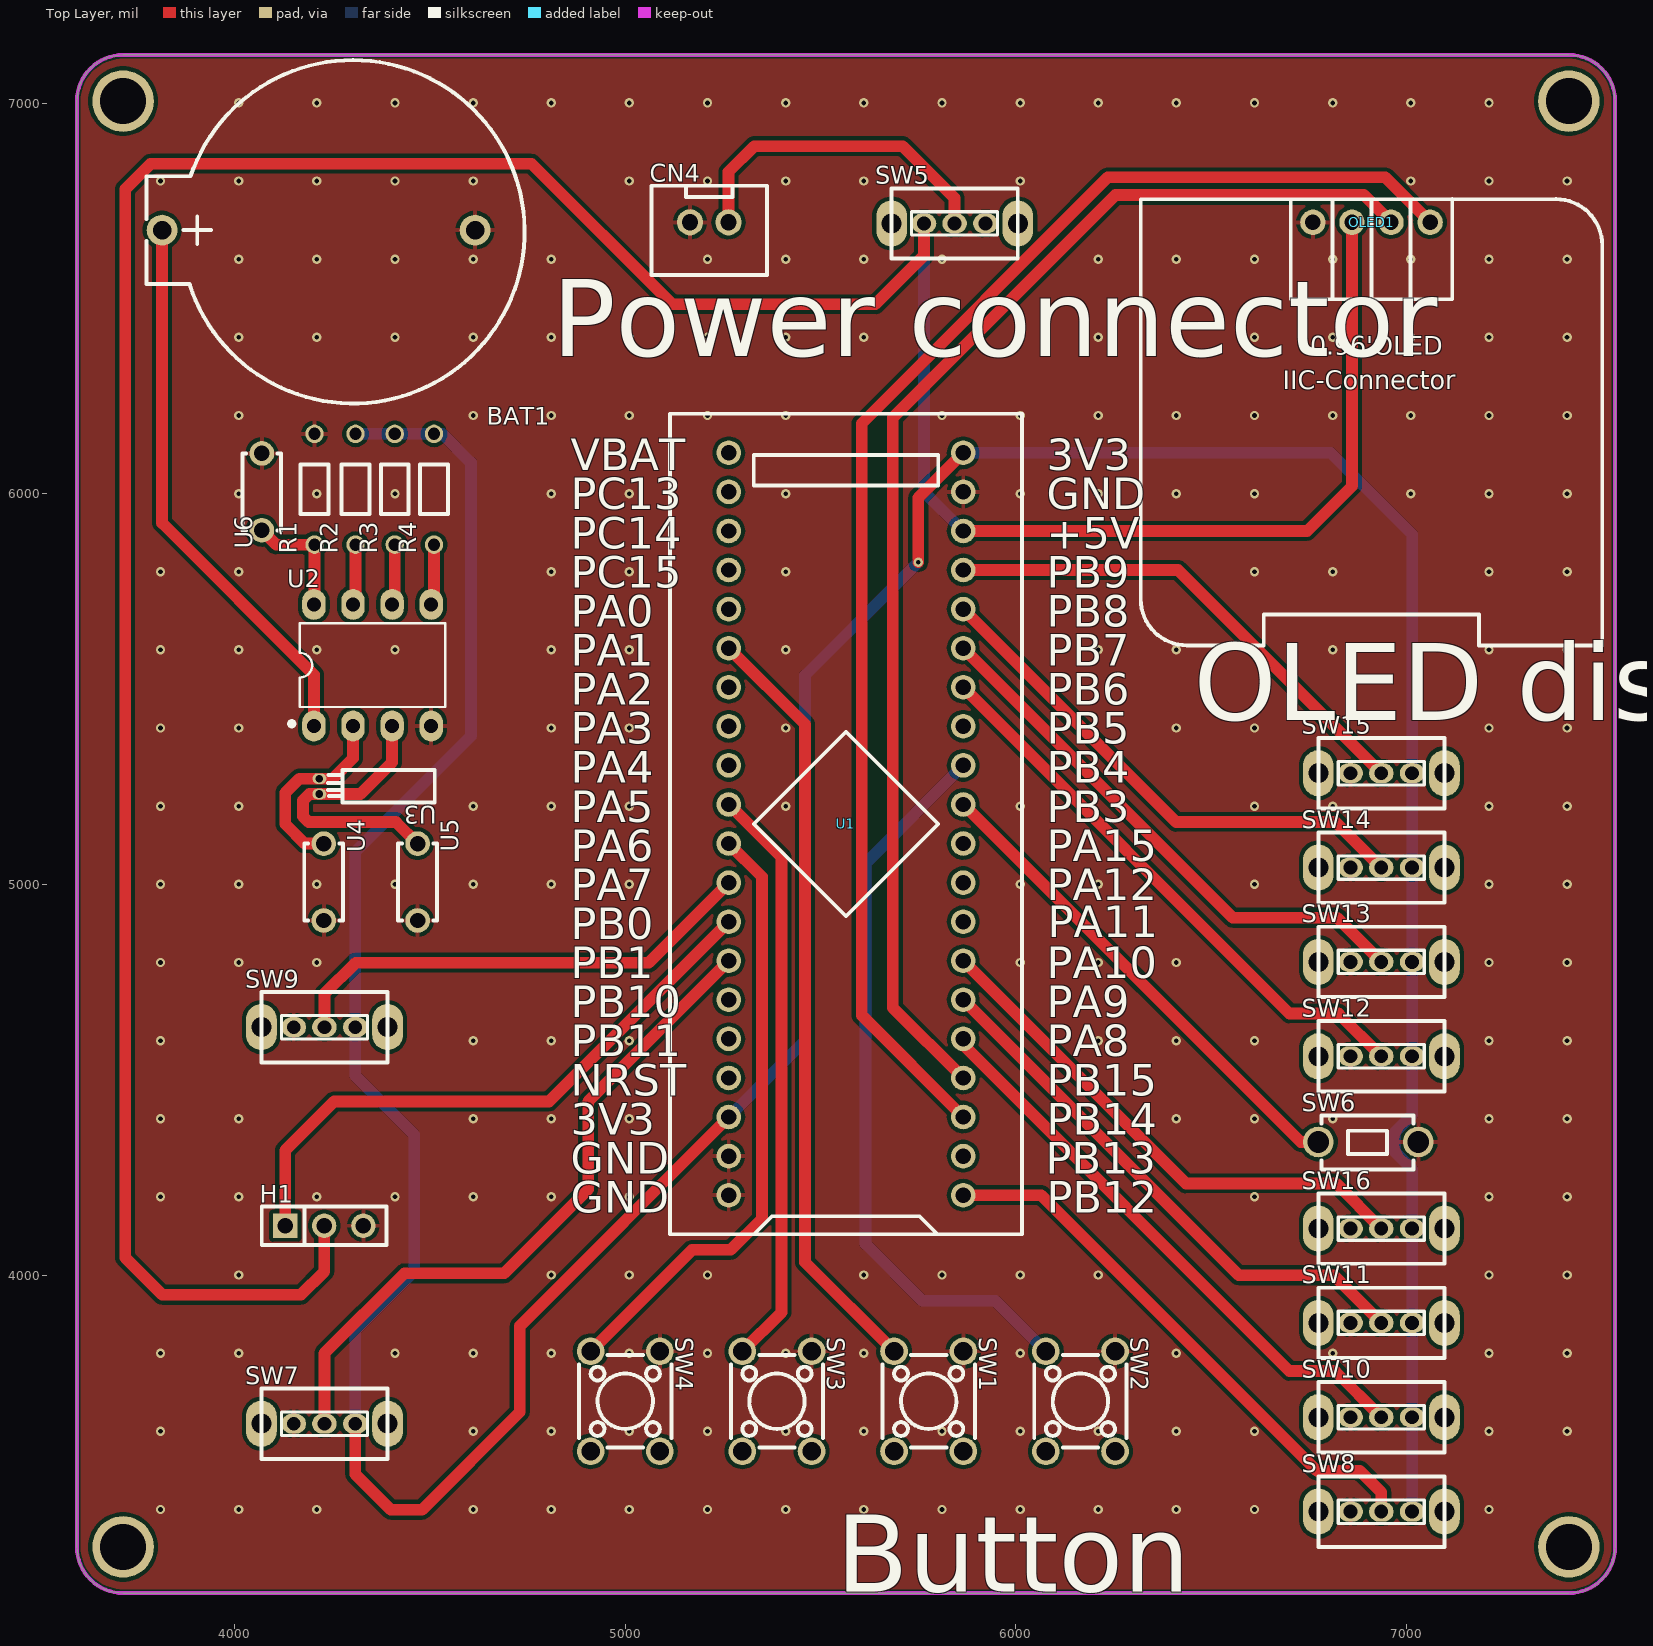
[diagram p0: Top Layer view]
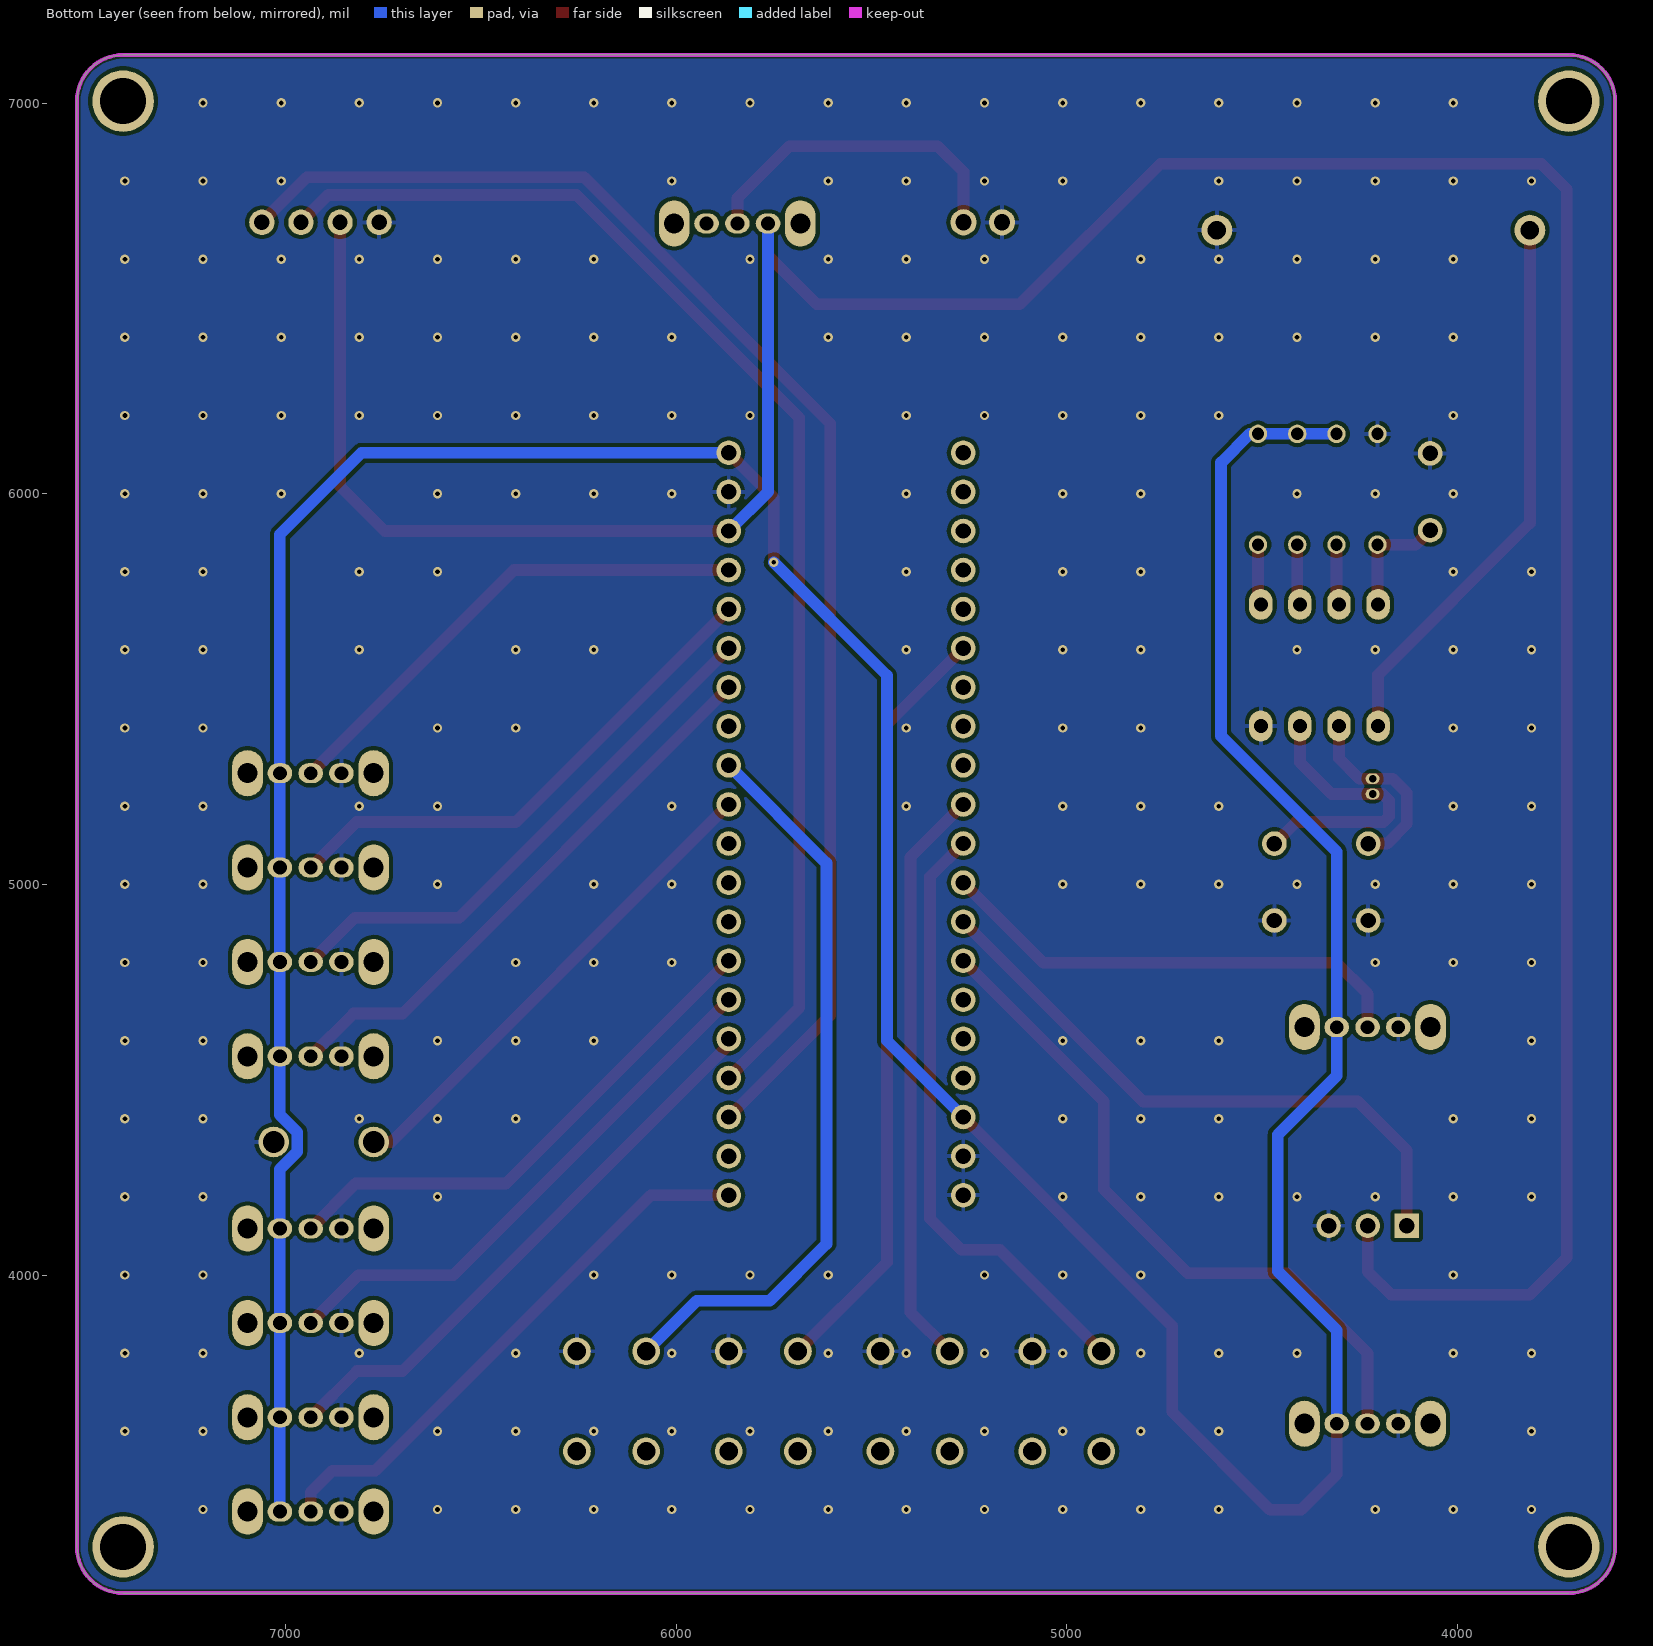
[diagram p1: Bottom Layer view, seen from below]
# Altium PCB MISC51813.pcbdoc
Units mil, origin at the board's own origin, x right, y up, seen from the top; angles counter-clockwise.
Board outline 3937.01 x 3937.01 mil, 2 copper layers (Top Layer, Bottom Layer), stack 62.206 mil thick; 30 components, 45 nets, 152 pads, 235 vias.

## Layer stack, top to bottom
Top Solder Mask Layer: solder mask 0.394, Dk 3.3
Top Layer: signal copper 1.379
Dielectric1: surface 59.449, FR4, Dk 4.5
Bottom Layer: signal copper 1.378
Bottom Solder Mask Layer: solder mask 0.394, Dk 3.3

## Board outline
3714.61,7123.5 ccw(c3714.61,7005.39) 3596.5,7005.39 3596.5,3304.61 ccw(c3714.61,3304.61) 3714.61,3186.5 7415.39,3186.5 ccw(c7415.39,3304.61) 7533.5,3304.61 7533.5,7005.39 ccw(c7415.39,7005.39) 7415.39,7123.5 3714.61,7123.5

## Design rules (kind name [scope] priority, off if disabled: settings)
BoardOutlineClearance copperThickness2oz_1 [All] p2 off: genericclearance=7.99 ignorepadtopadclearanceinfootprint=FALSE except(0: Arc-SplitContinuation Track-SplitContinuation SMDPad-SplitContinuation THPad-SplitContinuation Via-SplitContinuation Fill-SplitContinuation Region-SplitContinuation Poly-SplitContinuation Text-SplitContinuation Hole-SplitContinuation; 5.98: Arc-CutoutEdge Track-CutoutEdge SMDPad-CutoutEdge THPad-CutoutEdge Via-CutoutEdge Text-CutoutEdge; 6.9: Hole-OutlineEdge Hole-CutoutEdge; 10: Poly-OutlineEdge Poly-CutoutEdge; 11.81: Arc-OutlineEdge Track-OutlineEdge SMDPad-OutlineEdge THPad-OutlineEdge Via-OutlineEdge Fill-OutlineEdge Region-OutlineEdge Text-OutlineEdge Fill-CutoutEdge Region-CutoutEdge)
BoardOutlineClearance Plane_innerPlane_1 [All] p4 off: genericclearance=4.02 ignorepadtopadclearanceinfootprint=FALSE except(0: Arc-SplitContinuation Track-SplitContinuation SMDPad-SplitContinuation THPad-SplitContinuation Via-SplitContinuation Fill-SplitContinuation Region-SplitContinuation Poly-SplitContinuation Text-SplitContinuation Hole-SplitContinuation; 5.98: Arc-CutoutEdge Track-CutoutEdge SMDPad-CutoutEdge THPad-CutoutEdge Via-CutoutEdge Text-CutoutEdge; 6.9: Hole-OutlineEdge Hole-CutoutEdge; 10: Poly-OutlineEdge Poly-CutoutEdge; 11.81: Arc-OutlineEdge Track-OutlineEdge SMDPad-OutlineEdge THPad-OutlineEdge Via-OutlineEdge Fill-OutlineEdge Region-OutlineEdge Text-OutlineEdge Fill-CutoutEdge Region-CutoutEdge)
BoardOutlineClearance Copper_copperRegion_1 [All] p6 off: genericclearance=4.02 ignorepadtopadclearanceinfootprint=FALSE except(0: Arc-SplitContinuation Track-SplitContinuation SMDPad-SplitContinuation THPad-SplitContinuation Via-SplitContinuation Fill-SplitContinuation Region-SplitContinuation Poly-SplitContinuation Text-SplitContinuation Hole-SplitContinuation; 5.98: Arc-CutoutEdge Track-CutoutEdge SMDPad-CutoutEdge THPad-CutoutEdge Via-CutoutEdge Text-CutoutEdge; 6.9: Hole-OutlineEdge Hole-CutoutEdge; 10: Poly-OutlineEdge Poly-CutoutEdge; 11.81: Arc-OutlineEdge Track-OutlineEdge SMDPad-OutlineEdge THPad-OutlineEdge Via-OutlineEdge Fill-OutlineEdge Region-OutlineEdge Text-OutlineEdge Fill-CutoutEdge Region-CutoutEdge)
BoardOutlineClearance copperThickness1oz_1 [All] p8: genericclearance=4.02 ignorepadtopadclearanceinfootprint=FALSE except(0: Arc-SplitContinuation Track-SplitContinuation SMDPad-SplitContinuation THPad-SplitContinuation Via-SplitContinuation Fill-SplitContinuation Region-SplitContinuation Poly-SplitContinuation Text-SplitContinuation Hole-SplitContinuation; 5.98: Arc-CutoutEdge Track-CutoutEdge SMDPad-CutoutEdge THPad-CutoutEdge Via-CutoutEdge Text-CutoutEdge; 6.9: Hole-OutlineEdge Hole-CutoutEdge; 10: Poly-OutlineEdge Poly-CutoutEdge; 11.81: Arc-OutlineEdge Track-OutlineEdge SMDPad-OutlineEdge THPad-OutlineEdge Via-OutlineEdge Fill-OutlineEdge Region-OutlineEdge Text-OutlineEdge Fill-CutoutEdge Region-CutoutEdge)
Clearance copperThickness2oz [All] p1 off: gap=7.99 ignorepadtopadclearanceinfootprint=FALSE except(5.98: SMDPad-Track SMDPad-SMDPad THPad-Track SMDPad-THPad THPad-THPad Track-Via SMDPad-Via THPad-Via Via-Via Fill-SMDPad Region-SMDPad Fill-THPad Region-THPad Fill-Via Region-Via Fill-Fill Fill-Region Region-Region Arc-Track Arc-SMDPad Arc-THPad Arc-Via Fill-Arc Region-Arc Arc-Arc Text-Track SMDPad-Text Text-THPad Text-Via Fill-Text Region-Text Arc-Text Text-Text; 6.9: Hole-Track Hole-SMDPad Hole-THPad Hole-Via Fill-Hole Region-Hole Hole-Arc Hole-Text; 10: Poly-Track Poly-SMDPad Poly-THPad Poly-Via Poly-Fill Poly-Region Poly-Poly Poly-Arc Poly-Text Poly-Hole; 11.81: Fill-Track Region-Track)
Clearance Plane_innerPlane [All] p3 off: gap=4.02 ignorepadtopadclearanceinfootprint=FALSE except(5.98: SMDPad-Track SMDPad-SMDPad THPad-Track SMDPad-THPad THPad-THPad Track-Via SMDPad-Via THPad-Via Via-Via Fill-SMDPad Region-SMDPad Fill-THPad Region-THPad Fill-Via Region-Via Fill-Fill Fill-Region Region-Region Arc-Track Arc-SMDPad Arc-THPad Arc-Via Fill-Arc Region-Arc Arc-Arc Text-Track SMDPad-Text Text-THPad Text-Via Fill-Text Region-Text Arc-Text Text-Text; 6.9: Hole-Track Hole-SMDPad Hole-THPad Hole-Via Fill-Hole Region-Hole Hole-Arc Hole-Text; 10: Poly-Track Poly-SMDPad Poly-THPad Poly-Via Poly-Fill Poly-Region Poly-Poly Poly-Arc Poly-Text Poly-Hole; 11.81: Fill-Track Region-Track)
Clearance Copper_copperRegion [All] p5 off: gap=4.02 ignorepadtopadclearanceinfootprint=FALSE except(5.98: SMDPad-Track SMDPad-SMDPad THPad-Track SMDPad-THPad THPad-THPad Track-Via SMDPad-Via THPad-Via Via-Via Fill-SMDPad Region-SMDPad Fill-THPad Region-THPad Fill-Via Region-Via Fill-Fill Fill-Region Region-Region Arc-Track Arc-SMDPad Arc-THPad Arc-Via Fill-Arc Region-Arc Arc-Arc Text-Track SMDPad-Text Text-THPad Text-Via Fill-Text Region-Text Arc-Text Text-Text; 6.9: Hole-Track Hole-SMDPad Hole-THPad Hole-Via Fill-Hole Region-Hole Hole-Arc Hole-Text; 10: Poly-Track Poly-SMDPad Poly-THPad Poly-Via Poly-Fill Poly-Region Poly-Poly Poly-Arc Poly-Text Poly-Hole; 11.81: Fill-Track Region-Track)
Clearance copperThickness1oz [All] p7: gap=4.02 ignorepadtopadclearanceinfootprint=FALSE except(5.98: SMDPad-Track SMDPad-SMDPad THPad-Track SMDPad-THPad THPad-THPad Track-Via SMDPad-Via THPad-Via Via-Via Fill-SMDPad Region-SMDPad Fill-THPad Region-THPad Fill-Via Region-Via Fill-Fill Fill-Region Region-Region Arc-Track Arc-SMDPad Arc-THPad Arc-Via Fill-Arc Region-Arc Arc-Arc Text-Track SMDPad-Text Text-THPad Text-Via Fill-Text Region-Text Arc-Text Text-Text; 6.9: Hole-Track Hole-SMDPad Hole-THPad Hole-Via Fill-Hole Region-Hole Hole-Arc Hole-Text; 10: Poly-Track Poly-SMDPad Poly-THPad Poly-Via Poly-Fill Poly-Region Poly-Poly Poly-Arc Poly-Text Poly-Hole; 11.81: Fill-Track Region-Track)
DiffPairsRouting differentialPair [All] p1: maxlimit=6 minlimit=6 mostfreqgap=6 toplayer_minwidth=5 toplayer_prefwidth=10 toplayer_maxwidth=100 toplayer_mingap=6 toplayer_prefgap=6 toplayer_maxgap=6 bottomlayer_minwidth=5 bottomlayer_prefwidth=10 bottomlayer_maxwidth=100 bottomlayer_mingap=6 bottomlayer_prefgap=6 bottomlayer_maxgap=6 maxuncoupledlength=10
HoleToHoleClearance otherClearance [All] p1: gap=11.81 allowstackedmicrovias=TRUE
Length netLength [All] p1: minlimit=0 maxlimit=0
PasteMaskExpansion pasteMaskExpansion [All] p1: expansion=0
PlaneConnect innerPlane [All] p1: planeconnectstyle=Relief reliefexpansion=20 reliefentries=4 reliefconductorwidth=10 reliefairgap=10
PolygonConnect copperRegion [All] p1: connectstyle=Relief reliefconductorwidth=10 reliefentries=4 polygonreliefangle="90 Angle" airgapwidth=10 via.connectstyle=Relief via.reliefconductorwidth=10 via.reliefentries=4 via.polygonreliefangle="90 Angle" via.airgapwidth=10
RoutingVias viaSize [All] p1: holewidth=12.01 width=24.02 viastyle="Through Hole" minholewidth=11.81 minwidth=19.68 maxholewidth=248.03 maxwidth=393.7
SolderMaskExpansion solderMaskExpansion [IsVia] p1: expansion=-1000 istentingtop=TRUE
SolderMaskExpansion solderMaskExpansion [All] p2: expansion=2 istentingtop=FALSE
Width copperThickness2oz_2 [All] p1 off: maxlimit=100 minlimit=8 preferedwidth=10
Width copperThickness1oz_2 [All] p2: maxlimit=100 minlimit=5 preferedwidth=10

## Components (designator, comment, footprint, x,y, rotation, side; value= is the part's Value field where it differs from the comment)
BAT1 "CR2032-2-1" BAT-TH_CR2032-2-1 4215,6675 r180 top
CN4 "XH2.54*2P_through-hole" CONN-TH_2P-P2.50-XH2.54-2P 5215,6695 r0 top
H1 "" HDR-TH_3P-P2.54-V-F 4229.55,4126.75 r0 top
OLED1 "" 0.96OLED_4P 6910,6695 r0 top
R1 "10kΩ" Res_1/8W 4207.19,6011.78 r90 top
R2 "10kΩ" Res_1/8W 4312.02,6011.78 r90 top
R3 "10kΩ" Res_1/8W 4412.5,6011.78 r90 top
R4 "10kΩ" Res_1/8W 4512.99,6011.78 r90 top
SW1 "" SW-TH_4P-L6.0-W6.0-P4.50-LS6.5 5776.67,3677.47 r270 top
SW2 "" SW-TH_4P-L6.0-W6.0-P4.50-LS6.5 6165,3677.47 r270 top
SW3 "" SW-TH_4P-L6.0-W6.0-P4.50-LS6.5 5388.33,3677.47 r270 top
SW4 "" SW-TH_4P-L6.0-W6.0-P4.50-LS6.5 5000,3677.47 r270 top
SW5 "" 拨动开关 5837.9,6692.05 r0 top
SW6 "" Key_TH_3.5x6x4.3 6895.34,4341.1 r0 top
SW7 "" 拨动开关 4225,3620 r0 top
SW8 "" 拨动开关 6930,3395 r0 top
SW9 "" 拨动开关 4225,4635 r0 top
SW10 "" 拨动开关 6930,3636.53 r0 top
SW11 "" 拨动开关 6930,3878.05 r0 top
SW12 "" 拨动开关 6930,4560.43 r0 top
SW13 "" 拨动开关 6930,4801.95 r0 top
SW14 "" 拨动开关 6930,5043.48 r0 top
SW15 "" 拨动开关 6930,5285 r0 top
SW16 "" 拨动开关 6930,4119.57 r0 top
U1 "STM32F103C8T6-Card" CONN-TH_L53.3-W22.9_STM32F103C8T6-CARD 5565,5155 r90 top
U2 "DS1302N(LX)" PDIP-8_L9.3-W6.4-P2.54-LS7.9-BL-1 4353.22,5561.4 r0 top
U3 "32.768kHz" CRYSTAL-TH_BD2.1-P0.70-D0.3 4217.19,5251.38 r180 top
U4 "30pF" CAP-TH_L5.0-W2.5-P5.00-D1.0 4228.48,5006.4 r270 top
U5 "30pF" CAP-TH_L5.0-W2.5-P5.00-D1.0 4468.48,5006.4 r270 top
U6 "1nF" CAP-TH_L5.0-W2.5-P5.00-D1.0 4070,6005 r270 top

## Footprints (in the part's own frame and the unit in brackets; to place one, negate y for a bottom-side part, rotate by r counter-clockwise, add the part's x,y. Pads: shape width x height; smd on the part's side, far side on the other; paste and mask are expansions set on the pad)
0.96OLED_4P [mm]
  round 1.65 hole 1 copper offset 0,0: 1(-3.81,-0.001) 2(-1.27,0.002) 3(1.27,0.002) 4(3.81,0.002)
  silkscreen extent -15,-27.5 15,1.5
BAT-TH_CR2032-2-1 [mm]
  round 2 hole 1.2: 1(10.175,0) 2(-10.175,0)
  silkscreen extent -13.4,-11.05 11.17,11.26
CAP-TH_L5.0-W2.5-P5.00-D1.0 [mm]
  round 1.6 hole 1: 1(-2.5,0) 2(2.5,0)
  silkscreen extent -2.5,-1.27 2.5,1.25
CONN-TH_2P-P2.50-XH2.54-2P [mm]
  round 1.7 hole 1.05 paste+0 mask+0.05: 1(1.25,0) 2(-1.25,0)
  silkscreen extent -3.75,-3.42 3.75,2.37
CONN-TH_L53.3-W22.9_STM32F103C8T6-CARD [mm]
  round 1.6 hole 1: 1(-24.13,-7.62) 2(-21.59,-7.62) 3(-19.05,-7.62) 4(-16.51,-7.62) 5(-13.97,-7.62) 6(-11.43,-7.62) 7(-8.89,-7.62) 8(-6.35,-7.62) 9(-3.81,-7.62) 10(-1.27,-7.62) 11(1.27,-7.62) 12(3.81,-7.62) 13(6.35,-7.62) 14(8.89,-7.62) 15(11.43,-7.62) 16(13.97,-7.62) 17(16.51,-7.62) 18(19.05,-7.62) 19(21.59,-7.62) 20(24.13,-7.62) 21(24.13,7.62) 22(21.59,7.62) 23(19.05,7.62) 24(16.51,7.62) 25(13.97,7.62) 26(11.43,7.62) 27(8.89,7.62) 28(6.35,7.62) 29(3.81,7.62) 30(1.27,7.62) 31(-1.27,7.62) 32(-3.81,7.62) 33(-6.35,7.62) 34(-8.89,7.62) 35(-11.43,7.62) 36(-13.97,7.62) 37(-16.51,7.62) 38(-19.05,7.62) 39(-21.59,7.62) 40(-24.13,7.62)
  silkscreen extent -26.67,-11.43 26.67,11.43
CRYSTAL-TH_BD2.1-P0.70-D0.3 [mm]
  oval 0.9x0.7 hole 0.5 paste+0 mask+0.05: 1(0,0.5) 2(0,-0.5)
  silkscreen extent -7.5,-1.05 -0.57,1.05
HDR-TH_3P-P2.54-V-F [mil]
  rect 62x62 hole 40.16: 1(-100,0)
  round 62 hole 40.16: 2(0,0) 3(100,0)
  silkscreen extent -160,-49 160,49
Key_TH_3.5x6x4.3 [mil]
  round 78.7 hole 55.1 paste+0 mask+2: A(-121.44,0) B(134.46,0)
  silkscreen extent -114,-70 123,68
PDIP-8_L9.3-W6.4-P2.54-LS7.9-BL-1 [mm]
  oval 1.524x2 hole 0.9: 1(-3.81,-3.95) 2(-1.27,-3.95) 3(1.27,-3.95) 4(3.81,-3.95) 5(3.81,3.95) 6(1.27,3.95) 7(-1.27,3.95) 8(-3.81,3.95)
  silkscreen extent -5.4,-3.95 4.73,2.72
Res_1/8W [mil]
  round 47.2 hole 31.5 paste+0 mask+2: 1(-141.7,2.48) 2(141.7,2.48)
  silkscreen extent -63,-33 63,38
SW-TH_4P-L6.0-W6.0-P4.50-LS6.5 [mm]
  round 1.8 hole 1.2: 1(-3.25,2.25) 2(3.25,2.25) 3(-3.25,-2.25) 4(3.25,-2.25)
  silkscreen extent -3,-3 3,3
拨动开关 [mil]
  oval 63x51.2 hole 35.4 paste+0 mask+2: 1(-73.4,0) 2(5,0) 3(84,0)
  oval 78.7x118.1 hole 51.2 paste+0 mask+2: 4(166.7,0) 5(-156.1,0)
  silkscreen extent -156,-90 167,90

## Free pads (board coordinates)
  round 157.48 hole 118.11: 1(3714.61,7005.39) 1(3714.61,3304.61) 1(7415.39,7005.39) 1(7415.39,3304.61)

## Via types
v1: diameter 24.02, hole 12, Top Layer to Bottom Layer, 235 vias

## Nets (pads, with @x,y where several pads share a name; then routed paths per layer and width w, separated by ;. In a path a pad name is that pad's centre, name@x,y a point inside that pad or via, vN(x,y) a via of type N, cw(c..) or ccw(c..) an arc to the next point about the centre after c; other vN are vias at no path point)
$1N17118: CN4.1 SW5.2 | length 855.2
  Top Layer w30: CN4.1 5264.22,6824.22 5330,6890 5710,6890 5842.9,6757.1 SW5.2
$1N17188: U2.2 U3.2 U4.1 | length 491.7
  Top Layer w30: U4.1 4180.17,5104.83 4130,5155 4130,5235 4166.06,5271.06 U3.2 4251.06,5271.06 4303.22,5323.22 U2.2
$1N17189: U2.3 U3.1 U5.1 | length 724.1
  Top Layer w30: U2.3 4403.22,5313.22 4321.69,5231.69 U3.1 4191.69,5231.69 4175,5215 4175,5175 4190,5160 4413.31,5160 U5.1
$1N17190: BAT1.1 U2.1 | length 1430.2
  Top Layer w30: BAT1.1 3814.41,5925.59 4203.22,5536.78 U2.1
$1N17194: R1.1 U2.8 U6.2 | length 303.6
  Top Layer w30: U6.2 4106.49,5870.08 R1.1 4204.71,5718.41 U2.8
$1N17199: R4.1 U2.5 | length 156.2
  Top Layer w30: U2.5 4510.51,5724.2 R4.1
$1N17200: R3.1 U2.6 | length 156
  Top Layer w30: U2.6 4410.02,5723.72 R3.1
$1N17201: R2.1 U2.7 | length 155.8
  Top Layer w30: U2.7 4309.54,5723.23 R2.1
+5V: H1.2 OLED1.2 SW5.1 U1.18 | length 8326.8
  Top Layer w30: H1.2 4229.55,4009.55 4170,3950 3815,3950 3720,4045 3720,6780 3785,6845 4760,6845 5120,6485 5640,6485 5764.5,6609.5 SW5.1 ; U1.18 6745,5905 6860,6020 OLED1.2@6860,6695.05
  Bottom Layer w30: SW5.1 5764.5,6005.5 U1.18
GND: BAT1.2 CN4.2 H1.3 OLED1.1 R1.2 SW1.1 SW2.1 SW3.1 SW4.1 SW6.B SW7.1 SW8.1 SW9.1 SW10.1 SW11.1 SW12.1 SW13.1 SW14.1 SW15.1 SW16.1 U1.19 U1.39 U1.40 U2.4 U4.2 U5.2 U6.1
  other v1: 3810.6,3400.6 4010.6,3400.6 4210.6,3400.6 4610.6,3400.6 4810.6,3400.6 5010.6,3400.6 5210.6,3400.6 5410.6,3400.6 5610.6,3400.6 5810.6,3400.6 6010.6,3400.6 6210.6,3400.6 6410.6,3400.6 6610.6,3400.6 7210.6,3400.6 3810.6,3600.6 4610.6,3600.6 4810.6,3600.6 5010.6,3600.6 5210.6,3600.6 5410.6,3600.6 5610.6,3600.6 5810.6,3600.6 6010.6,3600.6 6210.6,3600.6 6410.6,3600.6 6610.6,3600.6 7210.6,3600.6 7410.6,3600.6 3810.6,3800.6 4010.6,3800.6 4410.6,3800.6 4610.6,3800.6 4810.6,3800.6 5010.6,3800.6 5210.6,3800.6 5410.6,3800.6 5610.6,3800.6 6010.6,3800.6 6410.6,3800.6 6810.6,3800.6 7210.6,3800.6 7410.6,3800.6 4010.6,4000.6 4810.6,4000.6 5010.6,4000.6 5210.6,4000.6 5610.6,4000.6 5810.6,4000.6 6010.6,4000.6 6210.6,4000.6 7210.6,4000.6 7410.6,4000.6 3810.6,4200.6 4010.6,4200.6 4210.6,4200.6 4410.6,4200.6 4610.6,4200.6 4810.6,4200.6 5010.6,4200.6 6610.6,4200.6 7210.6,4200.6 7410.6,4200.6 3810.6,4400.6 4010.6,4400.6 4610.6,4400.6 4810.6,4400.6 5010.6,4400.6 6410.6,4400.6 6610.6,4400.6 6810.6,4400.6 7210.6,4400.6 7410.6,4400.6 3810.6,4600.6 4610.6,4600.6 4810.6,4600.6 5010.6,4600.6 6210.6,4600.6 6410.6,4600.6 6610.6,4600.6 7210.6,4600.6 7410.6,4600.6 3810.6,4800.6 4010.6,4800.6 4210.6,4800.6 6010.6,4800.6 6210.6,4800.6 6410.6,4800.6 7210.6,4800.6 7410.6,4800.6 3810.6,5000.6 4010.6,5000.6 4210.6,5000.6 4410.6,5000.6 4610.6,5000.6 4810.6,5000.6 5010.6,5000.6 6010.6,5000.6 6210.6,5000.6 6610.6,5000.6 7210.6,5000.6 7410.6,5000.6 3810.6,5200.6 4010.6,5200.6 4610.6,5200.6 4810.6,5200.6 5010.6,5200.6 5410.6,5200.6 6010.6,5200.6 6610.6,5200.6 6810.6,5200.6 7210.6,5200.6 7410.6,5200.6 3810.6,5400.6 4010.6,5400.6 4810.6,5400.6 5010.6,5400.6 5410.6,5400.6 6410.6,5400.6 6610.6,5400.6 7210.6,5400.6 7410.6,5400.6 3810.6,5600.6 4010.6,5600.6 4210.6,5600.6 4410.6,5600.6 4810.6,5600.6 5010.6,5600.6 5410.6,5600.6 6210.6,5600.6 6410.6,5600.6 6810.6,5600.6 7210.6,5600.6 7410.6,5600.6 3810.6,5800.6 4010.6,5800.6 4810.6,5800.6 5010.6,5800.6 5410.6,5800.6 6610.6,5800.6 6810.6,5800.6 7210.6,5800.6 7410.6,5800.6 4010.6,6000.6 4210.6,6000.6 4410.6,6000.6 4810.6,6000.6 5010.6,6000.6 5410.6,6000.6 6010.6,6000.6 6210.6,6000.6 6410.6,6000.6 6610.6,6000.6 7010.6,6000.6 7210.6,6000.6 7410.6,6000.6 4010.6,6200.6 4610.6,6200.6 4810.6,6200.6 5010.6,6200.6 5210.6,6200.6 5410.6,6200.6 5810.6,6200.6 6010.6,6200.6 6210.6,6200.6 6410.6,6200.6 6610.6,6200.6 6810.6,6200.6 7010.6,6200.6 7210.6,6200.6 7410.6,6200.6 4010.6,6400.6 4210.6,6400.6 4410.6,6400.6 4610.6,6400.6 4810.6,6400.6 5010.6,6400.6 5210.6,6400.6 5410.6,6400.6 5610.6,6400.6 6010.6,6400.6 6210.6,6400.6 6410.6,6400.6 6610.6,6400.6 6810.6,6400.6 7010.6,6400.6 7210.6,6400.6 7410.6,6400.6 4010.6,6600.6 4210.6,6600.6 4410.6,6600.6 4610.6,6600.6 4810.6,6600.6 5210.6,6600.6 5410.6,6600.6 5610.6,6600.6 5810.6,6600.6 6210.6,6600.6 6410.6,6600.6 6610.6,6600.6 6810.6,6600.6 7010.6,6600.6 7210.6,6600.6 7410.6,6600.6 3810.6,6800.6 4010.6,6800.6 4210.6,6800.6 4410.6,6800.6 4610.6,6800.6 5010.6,6800.6 5210.6,6800.6 5410.6,6800.6 5610.6,6800.6 6010.6,6800.6 7010.6,6800.6 7210.6,6800.6 7410.6,6800.6 4010.6,7000.6 4210.6,7000.6 4410.6,7000.6 4610.6,7000.6 4810.6,7000.6 5010.6,7000.6 5210.6,7000.6 5410.6,7000.6 5610.6,7000.6 5810.6,7000.6 6010.6,7000.6 6210.6,7000.6 6410.6,7000.6 6610.6,7000.6 6810.6,7000.6 7010.6,7000.6 7210.6,7000.6
NRST: U1.37
PA0: U1.25
PA1: SW1.3 U1.26 | length 1974.8
  Top Layer w30: U1.26 5460,5410 5460,4033.51 SW1.3
PA2: U1.27
PA3: U1.28
PA4: U1.29
PA5: SW3.3 U1.30 | length 1497
  Top Layer w30: U1.30 5400,5070 5400,3905.67 SW3.3
PA6: SW4.3 U1.31 | length 1574.4
  Top Layer w30: SW4.3 5171,4065 5270,4065 5350,4145 5350,5020 U1.31
PA7: SW9.2 U1.32 | length 1238.1
  Top Layer w30: SW9.2 4230,4720 4310,4800 5060,4800 U1.32
PA8: SW10.2 U1.5 | length 1479.9
  Top Layer w30: U1.5 5865,4590 6700,3755 6816.52,3755 SW10.2
PA9: SW11.2 U1.6 | length 1412.5
  Top Layer w30: U1.6 6570,4000 6813.05,4000 SW11.2
PA10: SW16.2 U1.7 | length 1353.9
  Top Layer w30: U1.7 6435,4235 6819.57,4235 SW16.2
PA11: U1.8
PA12: U1.9
PA15: U1.10
PB0: H1.1 U1.33 | length 1570.8
  Top Layer w30: H1.1 4129.55,4319.55 4255,4445 4805,4445 U1.33
PB1: SW7.2 U1.34 | length 1763.1
  Top Layer w30: SW7.2 4230,3800 4435,4005 4690,4005 4905,4220 4905,4445 U1.34
PB3: SW6.A U1.11 | length 1266.7
  Top Layer w30: U1.11 6728.9,4341.1 SW6.A
PB4: SW2.3 U1.12 | length 1903.7
  Bottom Layer w30: U1.12 5615,5055 5615,4080 5760,3935 5946.84,3935 SW2.3
PB5: U1.13
PB6: SW12.2 U1.14 | length 1461.3
  Top Layer w30: U1.14 6700,4670 6825.43,4670 SW12.2
PB7: SW13.2 U1.15 | length 1402.6
  Top Layer w30: U1.15 6555,4915 6821.95,4915 SW13.2
PB8: SW14.2 U1.16 | length 1344
  Top Layer w30: U1.16 6410,5160 6818.48,5160 SW14.2
PB9: SW15.2 U1.17 | length 1285.4
  Top Layer w30: U1.17 6415,5805 SW15.2
PB10: U1.35
PB11: U1.36
PB12: SW8.2 U1.1 | length 1434.8
  Top Layer w30: U1.1 6065,4205 6770,3500 6880,3500 6935,3445 SW8.2
PB13: U1.2
PB14: OLED1.4 U1.3 | length 3646.3
  Top Layer w30: U1.3 5605,4665 5605,6180 6235,6810 6945.05,6810 OLED1.4@7060,6695.05
PB15: OLED1.3 U1.4 | length 3304.6
  Top Layer w30: U1.4 5685,4685 5685,6195 6255,6765 6890.05,6765 OLED1.3@6960,6695.05
PC13: U1.22
PC14: U1.23
PC15: U1.24
VBAT: U1.21
VCC: R2.2 R3.2 R4.2 SW7.3 SW8.3 SW9.3 SW10.3 SW11.3 SW12.3 SW13.3 SW14.3 SW15.3 SW16.3 U1.20 U1.38 | length 10423.4
  Top Layer w30: SW7.3 4309,3491 4400,3400 4480,3400 4730,3650 4730,3870 U1.38 ; v1(5750,5825) 5750,5990 U1.20
  Bottom Layer w30: SW7.3 4309,3859 4460,4010 4460,4360 4309,4511 SW9.3 4309,5084 4605,5380 4605,6080 4531.52,6153.48 R4.2 R3.2 R2.2 ; U1.38 5460,4600 5460,5535 v1(5750,5825) ; U1.20 6805,6105 7014,5896 SW15.3 SW14.3 SW13.3 SW12.3 7014,4410.63 6969.47,4366.09 6969.47,4316.11 7014,4271.57 SW16.3 SW11.3 SW10.3 SW8.3
pads on no net: SW1.2 SW1.4 SW2.2 SW2.4 SW3.2 SW3.4 SW4.2 SW4.4 SW5.3 SW5.4 SW5.5 SW7.4 SW7.5 SW8.4 SW8.5 SW9.4 SW9.5 SW10.4 SW10.5 SW11.4 SW11.5 SW12.4 SW12.5 SW13.4 SW13.5 SW14.4 SW14.5 SW15.4 SW15.5 SW16.4 SW16.5

## Polygon pours and split planes (outlines as drawn)
GND on Bottom Layer (solid, remove dead copper, pour order 2): 3525,7245 3525,3080 7700,3080 7700,7245
GND on Top Layer (solid, remove dead copper, pour order 2): 3000,7415 3000,3000 7930,3000 7930,7415

## Keep-outs
Board Outline Layer:
  the board outline again, w10

## Silkscreen, mask and mechanical layers (free items; w line width, h text height)
Top Silkscreen Layer:
  text "Power connector" at 4812.87,6351.57 h196.85
  text "VBAT" at 4860.95,6060 h80
  text "3V3" at 6079.16,6060 h80
  text "PC13" at 4860.95,5960 h80
  text "GND" at 6079.16,5960 h80
  text "PC14" at 4860.95,5860 h80
  text "+5V" at 6079.16,5860 h80
  text "PC15" at 4860.95,5760 h80
  text "PB9" at 6079.16,5760 h80
  text "PA0" at 4860.95,5660 h80
  text "PB8" at 6079.16,5660 h80
  text "PA1" at 4860.95,5560 h80
  text "PB7" at 6079.16,5560 h80
  text "PA2" at 4860.95,5460 h80
  text "PB6" at 6079.16,5460 h80
  text "OLED display" at 6455,5420 h196.85
  text "PA3" at 4860.95,5360 h80
  text "PB5" at 6079.16,5360 h80
  text "PA4" at 4860.95,5260 h80
  text "PB4" at 6079.16,5260 h80
  text "PA5" at 4860.95,5160 h80
  text "PB3" at 6079.16,5160 h80
  text "PA6" at 4860.95,5060 h80
  text "PA15" at 6079.16,5060 h80
  text "PA7" at 4860.95,4960 h80
  text "PA12" at 6079.16,4960 h80
  text "PA11" at 6080.95,4865 h80
  text "PB0" at 4860.95,4860 h80
  text "PB1" at 4860.95,4760 h80
  text "PA10" at 6079.16,4760 h80
  text "PB10" at 4860.95,4660 h80
  text "PA9" at 6079.16,4660 h80
  text "PB11" at 4860.95,4560 h80
  text "PA8" at 6079.16,4560 h80
  text "NRST" at 4860.95,4460 h80
  text "PB15" at 6079.16,4460 h80
  text "3V3" at 4860.95,4360 h80
  text "PB14" at 6079.16,4360 h80
  text "GND" at 4860.95,4260 h80
  text "PB13" at 6075.95,4260 h80
  text "GND" at 4860.95,4160 h80
  text "PB12" at 6079.16,4160 h80
  text "Button" at 5540,3190 h196.85